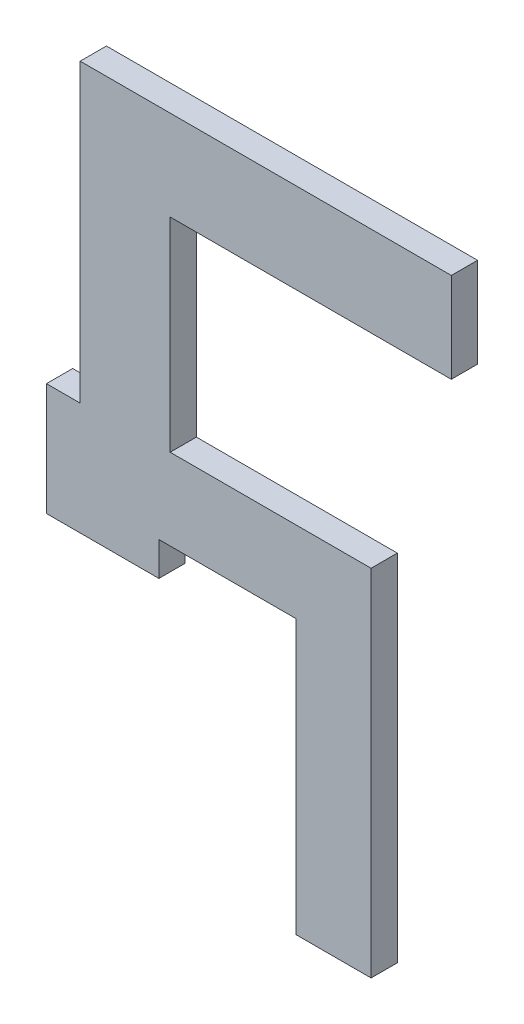
from build123d import *

# Parameters (mm, degrees)
BOSS_EXTRUDE1_DEPTH = 35


with BuildPart() as part:
    # Sketch1 → Boss-Extrude1 (new body)
    with BuildSketch(Plane.XY):
        Polygon((-495, -395), (-495, 0), (0, 0), (0, -120), (-375, -120), (-375, -391.71526804), (-107.021605816, -391.71526804), (-107.021605816, -865), (-207.021605816, -865), (-207.021605816, -500), (-390, -500), (-390, -545), (-540, -545), (-540, -395), align=None)
    extrude(amount=BOSS_EXTRUDE1_DEPTH)


solid = part.part
